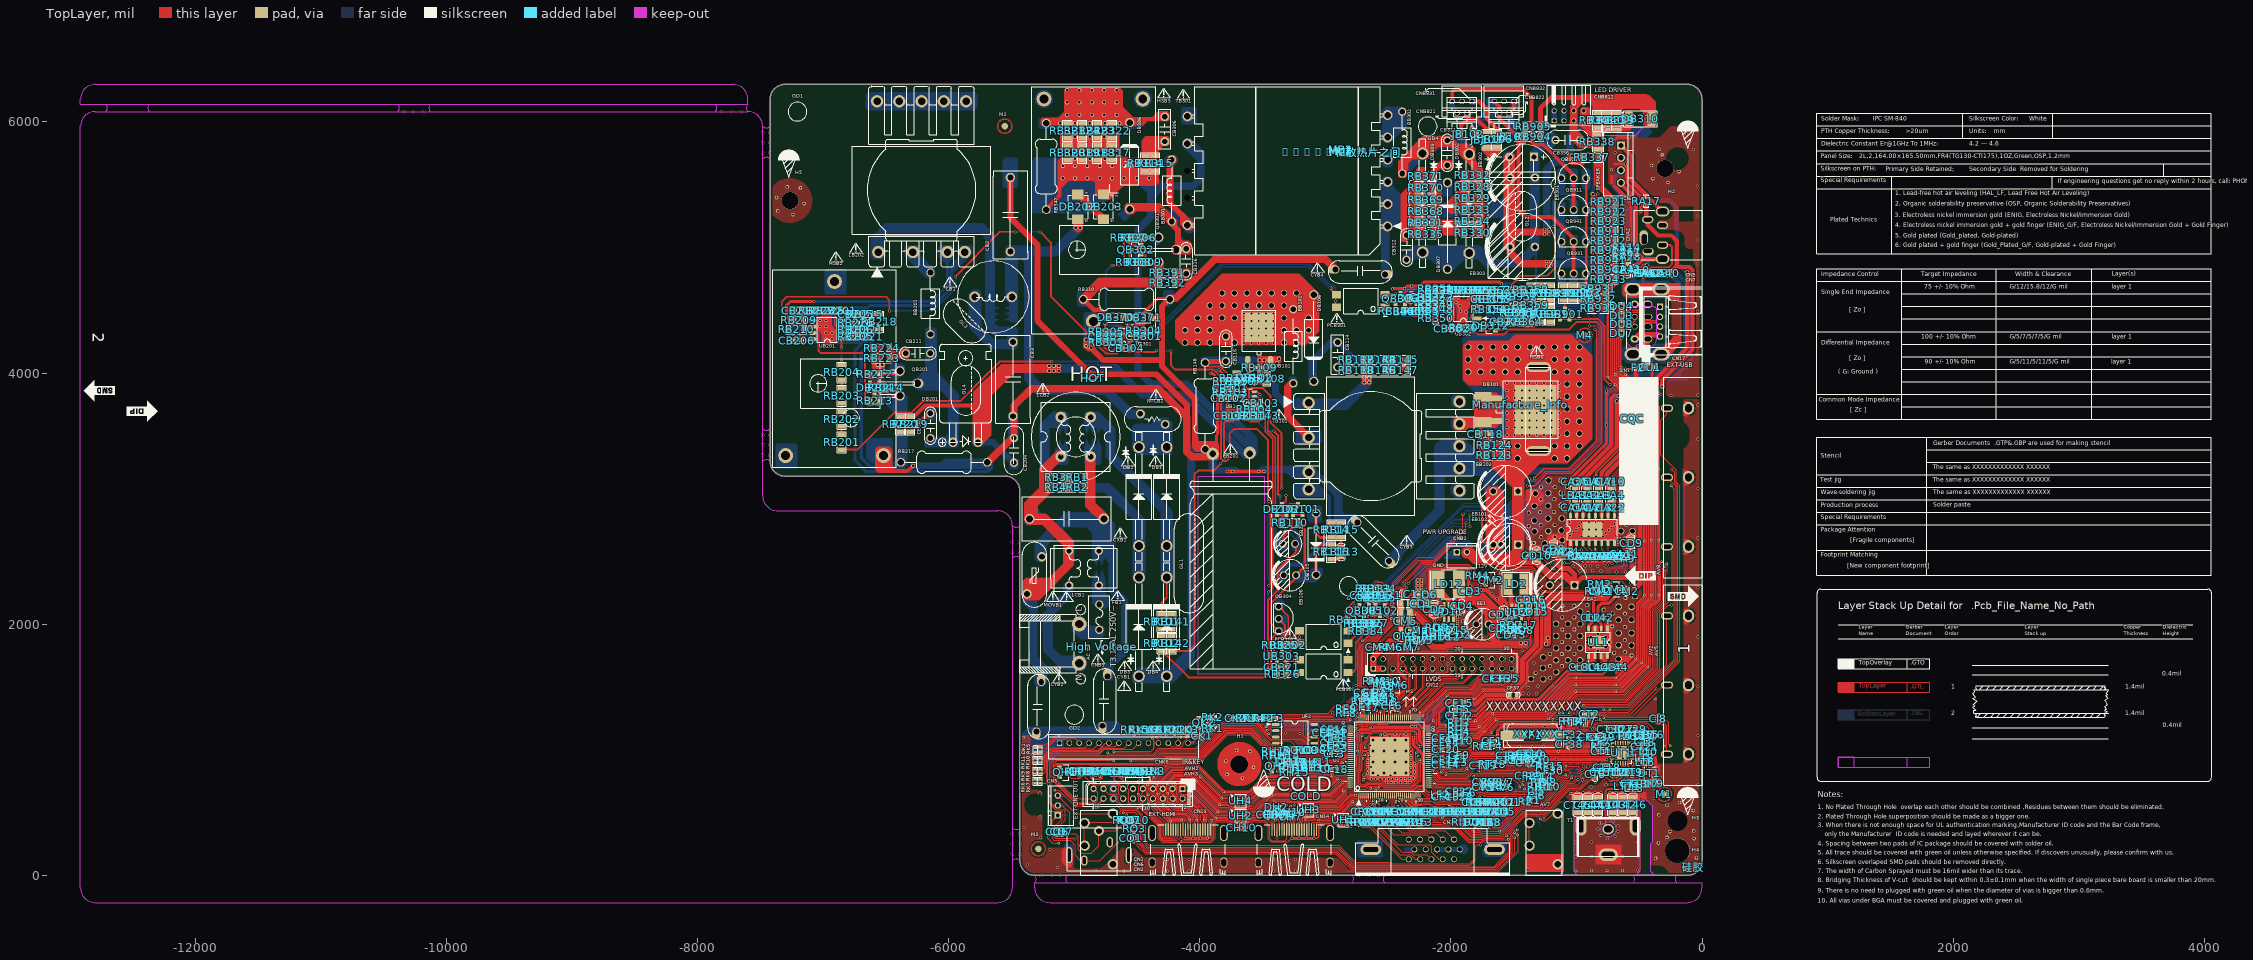
[diagram p0: TopLayer view]
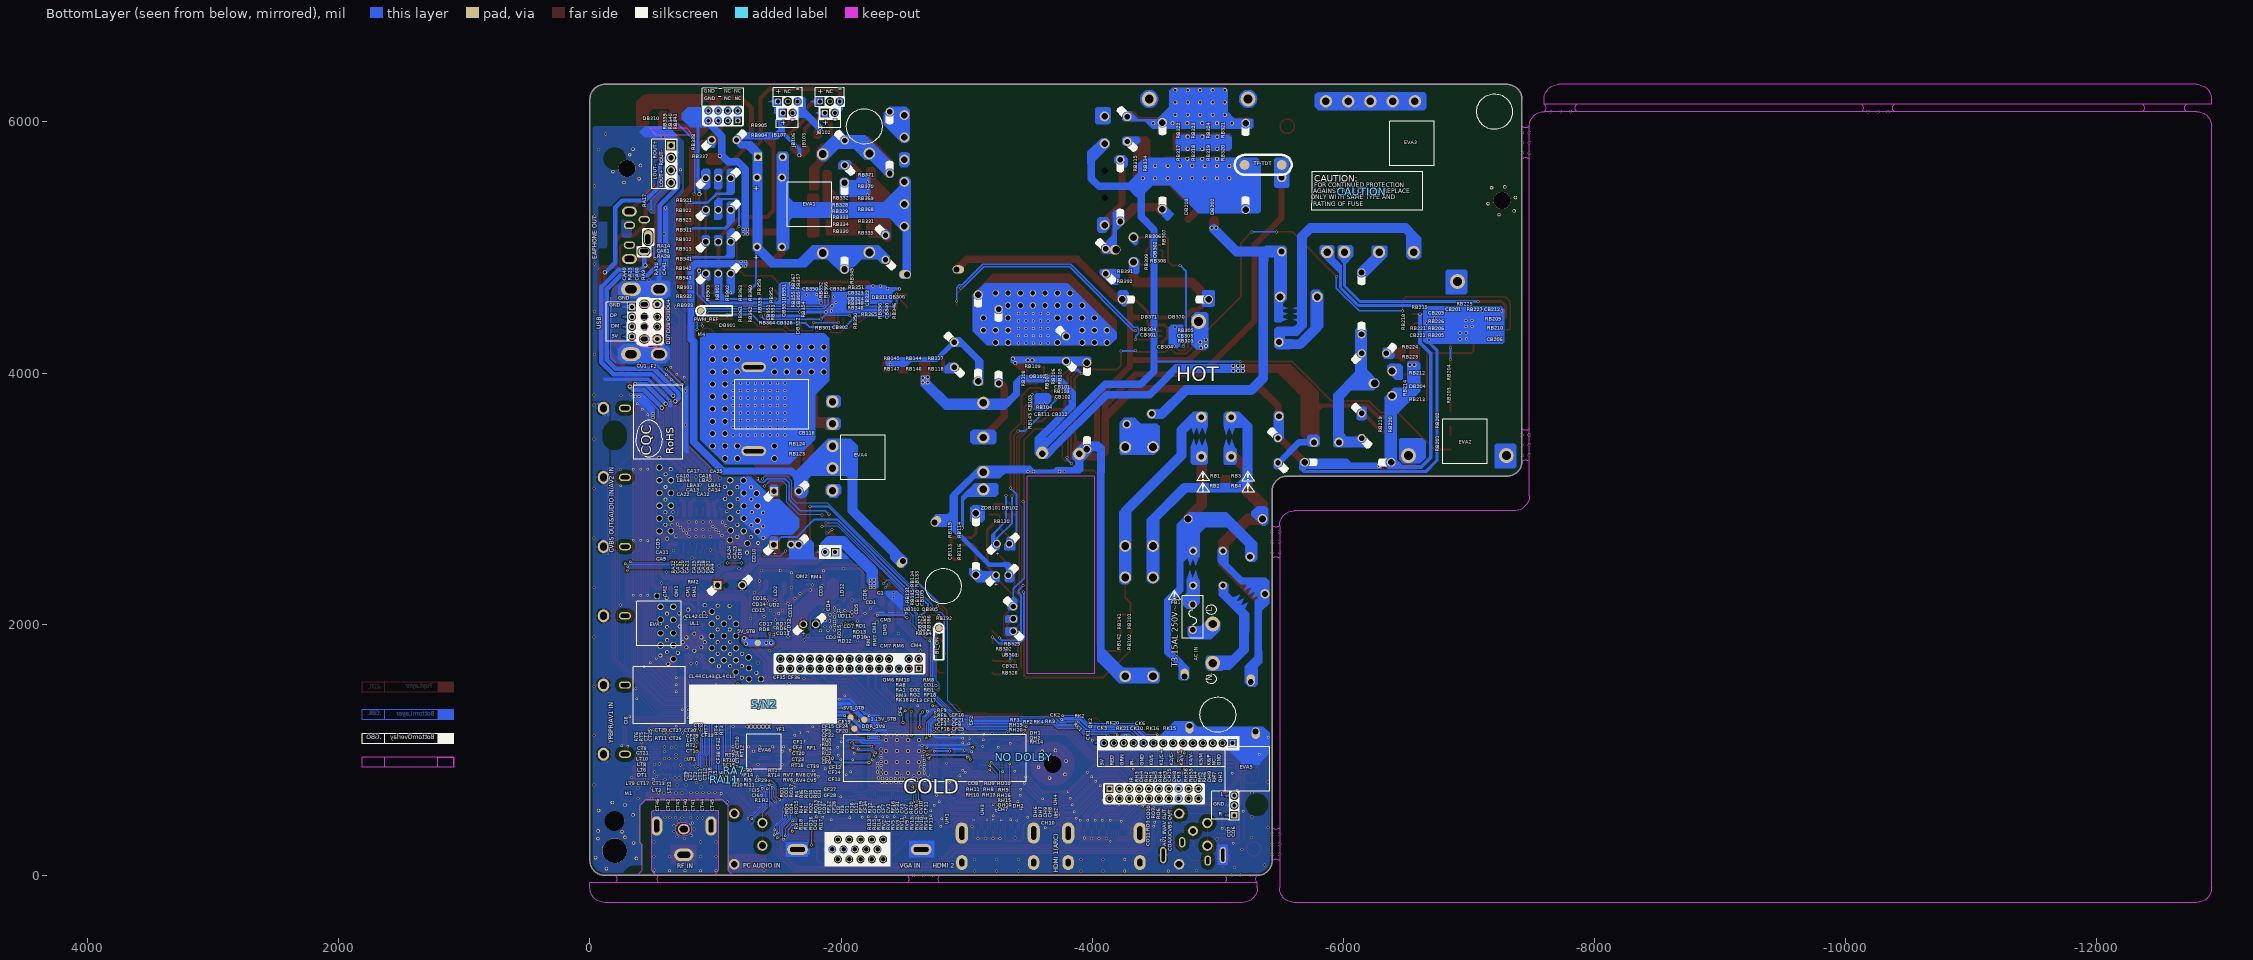
[diagram p1: BottomLayer view, seen from below]
# Altium PCB MISC84277.PcbDoc (part 1 of 15)
Units mil, origin at the board's own origin, x right, y up, seen from the top; angles counter-clockwise.
Board outline 7422.08 x 6299.21 mil, 2 copper layers (TopLayer, BottomLayer), stack 61.855 mil thick; 709 components, 395 nets, 2812 pads, 811 vias.

## Layer stack, top to bottom
TopSolder: solder mask 0.4, Solder Resist, Dk 3.5
TopLayer: signal copper 1.4
Dielectric1: core 59.055, FR-4, Dk 4.8
BottomLayer: signal copper 1.4
BottomSolder: solder mask 0.4, Solder Resist, Dk 3.5

## Board outline
-7304.33,3179.13 cw(c-7304.33,3297.24) -7422.44,3297.24 -7422.44,6181.1 cw(c-7304.33,6181.1) -7304.33,6299.21 -118.47,6299.21 cw(c-118.48,6181.1) -0.37,6181.1 -0.37,118.11 cw(c-118.48,118.11) -118.48,0 -5315.33,0 -5315.33,0.15 cw(c-5315.33,118.26) -5433.44,118.26 -5433.44,3061.02 ccw(c-5551.55,3061.02) -5551.55,3179.13

## Design rules (kind name [scope] priority, off if disabled: settings)
Clearance ■Poly_6.2mil [InPolygonClass('Poly_6.2mil') vs Not InPoly] p1: gap=6.2
Clearance ■KEEPOUT_18mil [(IsTrack Or IsArc) And (AsMM(Width) < 1) And IsKeepOut vs Not IsPad] p2: gap=18
Clearance ■HOT_7.2mm [InNetClass('HOT') vs InNetClass('All Nets') And (Not InNetClass('HOT'))] p3: gap=283.46
Clearance ■DFM_NPTH_10mil [IsPadHoleValid And (PadIsPlated=false) Or IsPad And (((AsMM(PadXSize_AllLayers) < 1) or (AsMM(PadYSize_AllLayers) < 1 ))) And IsKeepout vs Not IsPad] p4: gap=10
Clearance ■DFM_20mil [(IsTrack or IsArc or IsPad) And IsKeepOut vs IsTrack or IsArc or InPoly] p5: gap=20
Clearance ■PWR_A12_8mil [(InNetClass('PWR_A12_8mil') or InNet('*12V*') or InNet('*24V*') or InNet('*PVCC*') or InNet('*19V*') or InNet('*AMP*POWER*') or InNet('*AMP*VCC*') or InNet('*LNB*')) and Not IsPad vs Not InPoly] p6: gap=8
Clearance ■PS_L2All_3.2mm [InNet('L-1') vs InNet('*')] p7: gap=125.98
Clearance ■PS_L2LN_1.5mm [InNet('L') Or InNet('L-2') Or InNet('L-3') Or InNet('L-4') Or InNet('L-5') Or InNet('L-6') vs InNet('L-N') And Not(InNet('L') Or InNet('L-2') Or InNet('L-3') Or InNet('L-4') Or InNet('L-5') Or InNet('L-6'))] p8: gap=59.06
Clearance ■PS_N2LN_1.5mm [InNet('N') OR InNet('N-1') OR InNet('N-2') OR InNet('N-3') OR InNet('N-4') OR InNet('N-5') OR InNet('N-6') vs InNet('L-N') And Not (InNet('N') OR InNet('N-1') OR InNet('N-2') OR InNet('N-3') OR InNet('N-4') OR InNet('N-5') OR InNet('N-6'))] p9: gap=59.06
Clearance ■PS_L2LN_3mm [InNet('L') Or InNet('L-2') Or InNet('L-3') Or InNet('L-4') Or InNet('L-5') Or InNet('L-6') vs InNet('*') And Not (InNet('L-N') Or InNet('L') Or InNet('L-2') Or InNet('L-3') Or InNet('L-4') Or InNet('L-5') Or InNet('L-6') Or OnLayer('KeepOutLayer'))] p10: gap=118.11
Clearance ■PS_N2LN_3mm [InNet('N') OR InNet('N-1') OR InNet('N-2') OR InNet('N-3') OR InNet('N-4') OR InNet('N-5') OR InNet('N-6') vs InNet('*') And Not (InNet('L-N') Or InNet('N') OR InNet('N-1') OR InNet('N-2') OR InNet('N-3') OR InNet('N-4') OR InNet('N-5') OR InNet('N-6') Or OnLayer('KeepOutLayer'))] p11: gap=118.11
Clearance ■SIP2GND_8mil [HasFootprint('SIP*') vs InPoly] p12: gap=8
Clearance ■Poly_4mil [InPolygonClass('Poly_4mil') vs Not InPoly] p13: gap=4
Clearance ■Poly_5mil [InPolygonClass('Poly_5mil') vs Not InPoly] p14: gap=5
Clearance ■Poly_8mil [InPolygonClass('Poly_8mil') vs Not InPoly] p15: gap=8
Clearance ■ESD_10mil [HasFootprint('*IEC*') Or HasFootprint('*-F1*') Or HasFootprint('ANT-RF*')] p16: gap=10
Clearance ■ESD_20mil [HasFootprint('*SHIELD*')] p17: gap=20
Clearance ■C_RFGND_1.8mm [InNet('RFGND') vs Not (InNet('RF*IN*') OR InNet('NetCT40*'))] p18: gap=70.87
Clearance ■GND_12mil [InNet('GND') vs InPoly] p19: gap=12
Clearance ■ESD_30mil [(HasFootprint('SCART*') OR HasFootprint('AV*') OR HasFootprint('DB15*') OR HasFootprint('PHONE*')) vs OnBottomLayer] p20: gap=30
Clearance ■ESD_NT_30mil [HasFootprint('SCART*') Or HasFootprint('PHONE-HD-12') Or HasFootprint('PHONE-HD-17') Or HasFootprint('PHONE-HD-10') Or HasFootprint('PHONE-HD-26') vs InNet('GND') And OnTopLayer] p21: gap=30
Clearance ■DFM_TH_5mil [HasFootprint('GND') or HasFootprint('TP*') or HasFootprint('MARK*') or HasFootprint('SPARK_GAP') or HasFootprint('USB-HD-3-2') or HasFootprint('PHONE-HS-20') and Not IsRegion vs OnBottomlayer And IsPad OR IsPadHoleValid] p22: gap=5
Clearance ■DFM_HS60_5mil [InPadClass('HS60') vs InPadClass('HS60') OR IsPadHoleValid and not InPadClass('VIA5')] p23: gap=5
Clearance ■DFM_BCR_4mm [IsPadHoleValid vs IsBoardCutoutRegion] p24: gap=157.48
Clearance ■DFM_TH_4mm [OnBottomlayer And IsSMTPin vs IsPadHoleValid and not InPadClass('VIA5')] p25: gap=157.48
Clearance ■DFM_HS60_4mm [InPadClass('HS60') vs IsPad and OnBottomlayer] p26: gap=157.48
Clearance ■VIA2VIA_6.2mil [(IsVia OR InPadClass('VIA5')) And Not (IsVia And (AsMM(HoleDiameter) = 0.1)) vs (IsVia OR InPadClass('VIA5')) And Not (IsVia And (AsMM(HoleDiameter) = 0.1))] p27: gap=6.2
Clearance ■VIA2VIA_10.2mil [(IsVia OR InPadClass('VIA5')) And Not (IsVia And (AsMM(HoleDiameter) = 0.1)) vs (IsVia OR InPadClass('VIA5')) And Not (IsVia And (AsMM(HoleDiameter) = 0.1))] p28: gap=10.2
Clearance ■VIA2PAD_BGA_5mil [HasFootprint('BGA*') and IsPad vs (IsVia OR InPadClass('VIA5')) And Not (IsVia And (AsMM(HoleDiameter) = 0.1))] p29: gap=5
Clearance ■VIA2PAD_6mil [IsVia And Not (IsVia And (AsMM(HoleDiameter) = 0.1)) vs IsPad and Not HasFootprintPad('*','EPAD') and Not HasFootprintPad('*','257') and Not HasFootprintPad('TP','*') and Not HasFootprintPad  ('GND','JP*') and Not HasFootprintPad('LQFP216/0.4-2','217') and Not HasFootprintPad('QFP16*','17') and Not HasFootprintPad('QFN16*','17')  and Not HasFootprintPad('QFN20*','21') and Not HasFootprintPad('QFN24*','25') and Not HasFootprintPad( 'QFN24*','29') and Not  HasFootprintPad('QFN28*','29') and Not HasFootprintPad('QFN32*','33') and Not HasFootprintPad('QFN36*','37') and Not HasFootprintPad  ('QFN36*','0') and Not HasFootprintPad('QFN32*','0') and Not HasFootprintPad('QFN40*','41') and Not HasFootprintPad('QFN48*','49') and Not  HasFootprintPad('LQFP48/0.5-2','49') and Not HasFootprintPad('*SSOP32*','33') and Not HasFootprintPad('SOP8*','9') and Not HasFootprintPad  ('WSON8/1.27*','9') and Not HasFootprintPad('DFN10/0.5-1*','11') and Not HasFootprintPad('SON16/0.4','9') and Not HasFootprintPad  ('MSOP10/0.5-1','11') and Not HasFootprintPad('QFN56/0.5','57') and Not HasFootprintPad('LGA31/0.5','3*') and Not InPadClass('VIA_HS60')  and Not HasFootprintPad('TSSOP16/0.65-3','17') and Not HasFootprintPad('QFP128/0.5-2','129') and Not HasFootprintPad('QFP128/0.4-5','129')  and Not HasFootprintPad('PQFP48*','49') and Not HasFootprintPad('QFP156/0.4-1','157')] p30: gap=6
Clearance ■PAD2VIA5_6mil [IsPad And ((AsMM(PadXSize_AllLayers) < 2.5) or ((AsMM(PadYSize_AllLayers) < 2.5))) And Not InPadclass('HS60') vs InPadClass('VIA5')] p31: gap=6
Clearance "■12mil for Polygon" [InPoly] p32: gap=12
Clearance 8mil [All] p33 off: gap=8
Clearance 7mil [All] p34 off: gap=7
Clearance 6.2mil [All] p35 off: gap=6.2
Clearance 6mil [All] p36 off: gap=6
Clearance 5.8mil [All] p37 off: gap=5.8
Clearance 5mil [Not ((IsTrack Or IsArc) And (Layer = 'KeepOutLayer')) vs Not (IsPad or ((IsTrack Or IsArc) And (Layer = 'KeepOutLayer')))] p38: gap=5
Clearance 4.5mil [Not ((IsTrack Or IsArc) And (Layer = 'KeepOutLayer')) vs Not (IsPad or ((IsTrack Or IsArc) And (Layer = 'KeepOutLayer')))] p39 off: gap=4.5
Clearance "4mil for Minimum" [Not ((IsTrack Or IsArc) And (Layer = 'KeepOutLayer')) vs Not (IsPad or ((IsTrack Or IsArc) And (Layer = 'KeepOutLayer')))] p40 off: gap=4
ComponentClearance [All] p1 off: gap=0.1 collisioncheckmode=3 verticalgap=39.37 showdistances=FALSE
DiffPairsRouting DiffPair_USB_DiffPairsRouting [InDifferentialPairClass('USB')] p1: maxlimit=5 minlimit=4 mostfreqgap=5 toplayer_minwidth=15 toplayer_maxwidth=15 toplayer_prefwidth=15 bottomlayer_minwidth=15 bottomlayer_maxwidth=15 bottomlayer_prefwidth=15 maxuncoupledlength=200
DiffPairsRouting DiffPair_LVDS_DiffPairsRouting [InDifferentialPairClass('LVDS')] p2: maxlimit=5 minlimit=4 mostfreqgap=5 toplayer_minwidth=15 toplayer_maxwidth=15 toplayer_prefwidth=15 bottomlayer_minwidth=15 bottomlayer_maxwidth=15 bottomlayer_prefwidth=15 maxuncoupledlength=500
DiffPairsRouting DiffPair_HDMI_DiffPairsRouting [InDifferentialPairClass('HDMI')] p3: maxlimit=5 minlimit=4 mostfreqgap=5 toplayer_minwidth=15 toplayer_maxwidth=15 toplayer_prefwidth=15 bottomlayer_minwidth=15 bottomlayer_maxwidth=15 bottomlayer_prefwidth=15 maxuncoupledlength=200
DiffPairsRouting [All] p4: maxlimit=10 minlimit=10 mostfreqgap=10 toplayer_minwidth=15 toplayer_maxwidth=15 toplayer_prefwidth=15 bottomlayer_minwidth=15 bottomlayer_maxwidth=15 bottomlayer_prefwidth=15 maxuncoupledlength=500
FabricationTestPointUsage TestPointUsage [All] p1: valid=0 allowmultiple=FALSE
FabricationTestpoint Testpoint [All] p1: side=3 testpointundercomponent=TRUE minsize=40 maxsize=100 preferedsize=60 minholesize=20 maxholesize=40 preferedholesize=32 testpointgrid=1 allowsidetop=TRUE allowsidebottom=TRUE usegrid=TRUE gridtolerance=0.01
HoleSize HoleSize_VIA [ISVIA] p1 off: absolutevalues=TRUE maxlimit=23.62 minlimit=7.87 maxpercent=80.000 minpercent=20.000
HoleToHoleClearance Hole2Hole [All] p1 off: gap=18 allowstackedmicrovias=FALSE
MatchedLengths DiffPair_USB_MatchedLengths [InDifferentialPairClass('USB')] p1: tolerance=100 checknetsindiffpair=TRUE checkdiffpairvsdiffpair=TRUE checkothers=TRUE
MatchedLengths DiffPair_LVDS_MatchedLengths [InDifferentialPairClass('LVDS')] p2: tolerance=100 checknetsindiffpair=TRUE checkdiffpairvsdiffpair=TRUE checkothers=TRUE
MatchedLengths DiffPair_HDMI_MatchedLengths [InDifferentialPairClass('HDMI')] p3: tolerance=100 checknetsindiffpair=TRUE checkdiffpairvsdiffpair=TRUE checkothers=TRUE
MinimumAnnularRing [All] p1: minimumring=3.94
MinimumSolderMaskSliver [All] p1 off: minsoldermaskwidth=-1
NetAntennae [Not (HasFootprint('ANT-7') or HasFootprint('ANT-BLUECORE'))] p1: netantennaetolerance=40
PermittedLayers [All] p1: toplayerpermitted=TRUE bottomlayerpermitted=TRUE
PlaneClearance Plane_ESD_30mil [(HasFootprint('SCART*') OR HasFootprint('AV*') OR HasFootprint('DB15*') OR HasFootprint('PHONE*'))] p1: clearance=30
PlaneClearance [All] p2: clearance=9
PlaneConnect Plane2Via [IsVia or InPadClass('VIA5')] p1: planeconnectstyle=Direct reliefexpansion=20 reliefentries=4 reliefconductorwidth=10 reliefairgap=10
PlaneConnect PlaneConnect_PAD [HasFootprint('ASSE*') OR InPadclass('HS60')] p2: planeconnectstyle=Direct reliefexpansion=20 reliefentries=4 reliefconductorwidth=10 reliefairgap=10
PlaneConnect [All] p3: planeconnectstyle=Relief reliefexpansion=12 reliefentries=4 reliefconductorwidth=30 reliefairgap=12
PolygonConnect PourOverVia [IsVia vs IsPolygon] p1: connectstyle=Direct reliefconductorwidth=10 reliefentries=4 polygonreliefangle="90 Angle" airgapwidth=10
PolygonConnect VIA5_HS60 [InPadclass('HS60') or InPadClass('VIA5') vs IsPolygon] p2: connectstyle=Direct reliefconductorwidth=10 reliefentries=4 polygonreliefangle="90 Angle" airgapwidth=10
PolygonConnect Polygon_RFGND [InNet('RFGND')] p3: connectstyle=Direct reliefconductorwidth=10 reliefentries=4 polygonreliefangle="90 Angle" airgapwidth=10
PolygonConnect ESD_SCART [HasFootprint('SCART*') vs IsPolygon And onBottomlayer] p4: connectstyle=Direct reliefconductorwidth=30 reliefentries=4 polygonreliefangle="90 Angle" airgapwidth=10
PolygonConnect FH2Polygon [HasFootprint('ASSE*') or HasFootprint('DIODE-S0402') vs IsPolygon] p5: connectstyle=Direct reliefconductorwidth=10 reliefentries=4 polygonreliefangle="90 Angle" airgapwidth=10
PolygonConnect PWC1_2Polygon [(HasFootprint('*0805*') OR HasFootprint('*1206*')) vs IsPolygon] p6: connectstyle=Relief reliefconductorwidth=30 reliefentries=4 polygonreliefangle="90 Angle" airgapwidth=10
PolygonConnect PWC2_2Polygon [HasFootprint('*0603*') vs IsPolygon] p7: connectstyle=Relief reliefconductorwidth=25 reliefentries=4 polygonreliefangle="90 Angle" airgapwidth=10
PolygonConnect PWC3_2Polygon [HasFootprint('EC*') vs IsPolygon] p8: connectstyle=Relief reliefconductorwidth=35 reliefentries=4 polygonreliefangle="90 Angle" airgapwidth=10
PolygonConnect PWC2Polygon [(HasFootprint('SOT-89') OR HasFootprint('SOT-223') OR HasFootprint('TO-252') OR HasFootprint('TO-263') OR HasFootprint('DIODE') OR HasFootprint('SW-HS-2') OR HasFootprint('HDMI*') OR HasFootprint('SO-8B') OR HasFootprint('GND') OR HasFootprint('PHONE*') OR HasFootprint('DIP18/2.54-2') OR HasFootprint('DIP18/2.54-1') OR HasFootprint('UFL-R-SMT-1') OR HasFootprint('WIFI') OR HasFootprint('UM02BS') OR HasFootprint('*SCART*') OR HasFootprint('TSOT23-8/0.65') OR HasFootprint('*SOT-23-*') OR HasFootprint('SOP23-5-1') OR HasFootprint('SOP6/0.95') OR HasFootprint('M-WIFI-2-M603USA1') OR HasFootprint('M-MT7632U') OR HasFootprint('SOP8/1.27') OR HasFootprint('SOP8/1.27-3')) vs IsPolygon] p9: connectstyle=Direct reliefconductorwidth=35 reliefentries=4 polygonreliefangle="90 Angle" airgapwidth=10
PolygonConnect SMD2Polygon [IsSMTPin vs IsPolygon] p10: connectstyle=Relief reliefconductorwidth=12 reliefentries=4 polygonreliefangle="90 Angle" airgapwidth=10
PolygonConnect PTH2Polygon [IsThruPin vs IsPolygon] p11: connectstyle=Relief reliefconductorwidth=25 reliefentries=4 polygonreliefangle="90 Angle" airgapwidth=10
RoutingVias 0.6_0.4 [All] p1 off: holewidth=15.75 width=23.62 viastyle="Through Hole" minholewidth=15.75 minwidth=23.62 maxholewidth=15.75 maxwidth=23.62
RoutingVias 0.8_0.5 [All] p2 off: holewidth=19.68 width=31.5 viastyle="Through Hole" minholewidth=19.68 minwidth=31.5 maxholewidth=19.68 maxwidth=31.5
RoutingVias 0.5_0.3 [All] p3: holewidth=11.81 width=19.68 viastyle="Through Hole" minholewidth=11.81 minwidth=19.68 maxholewidth=11.81 maxwidth=19.68
RoutingVias 0.45_0.25 [All] p4 off: holewidth=9.84 width=17.72 viastyle="Through Hole" minholewidth=9.84 minwidth=17.72 maxholewidth=9.84 maxwidth=17.72
RoutingVias 0.4_0.2 [All] p5 off: holewidth=7.87 width=15.75 viastyle="Through Hole" minholewidth=7.87 minwidth=15.75 maxholewidth=7.87 maxwidth=15.75
RoutingVias 0.25_0.1 [All] p6 off: holewidth=3.94 width=9.84 viastyle="Through Hole" minholewidth=3.94 minwidth=9.84 maxholewidth=3.94 maxwidth=9.84
SMDNeckDown SMDNeckDown_Chip [HasFootprint('FFC*') or HasFootprint('QFP*') or HasFootprint('QFN*') or HasFootprint('HDMI*') or HasFootprint('BGA*')] p1: percent=100.000
SMDToCorner [All] p1 off: distance=40000
ShortCircuit ■ShortCircuit_ViaOnEpad [HasFootprintPad( '*','EPAD') vs IsVia AND InNet('*')] p1: allowed=TRUE
ShortCircuit ■ShortCircuit_JP [HasFootprintPad( 'GND','JP_1K') vs HasFootprintPad( 'GND','JP_2K')] p2: allowed=TRUE
ShortCircuit ■ShortCircuit_0402 [HasFootprintPad('R0402SC','1') Or HasFootprintPad('R0402SC','2') vs HasFootprintPad('R0402SC','3')] p3: allowed=TRUE
ShortCircuit ■ShortCircuit [InNet('*')] p4: allowed=FALSE
SilkToSilkClearance Silk2Silk [All] p1: silktosilkclearance=0.1
SilkToSolderMaskClearance SilkscreenOverComponentPads [IsText] p1: minsilkscreentomaskgap=0.1 clearancetoexposedcopper=TRUE
SolderMaskExpansion SolderMask_VIA [IsVia] p1: expansion=5.1
SolderMaskExpansion [All] p2: expansion=3
UnRoutedNet ■UnRoutedNet [All] p1:
ViasUnderSMD [All] p1: allowed=FALSE
Width DiffPair_USB_Width [InDifferentialPairClass('USB')] p1: maxlimit=11 minlimit=4 preferedwidth=11
Width DiffPair_LVDS_Width [InDifferentialPairClass('LVDS')] p2: maxlimit=7 minlimit=4 preferedwidth=7
Width DiffPair_HDMI_Width [InDifferentialPairClass('HDMI')] p3: maxlimit=7 minlimit=4 preferedwidth=7
Width [All] p4: maxlimit=250 minlimit=3 preferedwidth=8
16 further rules are at their usual default settings.

## Classes and differential pairs
net class HOT: 380V BRO BRO1 COMP CS D H L L-1 L-2 L-3 L-N N-1 N-2 N-3 NetBB101_2 NetBB201_1 NetBB201_2 NetBB301_1 NetCB3_1 NetCB101_1 NetCB102_1 NetCB103_1 NetCB111_2 NetCB113_1 NetCB113_2 NetCB114_1 NetCB114_2 NetCB116_1 NetCB201_2 NetCB206_2 NetCB209_1 NetCB211_2 NetCB212_1 NetCB221_2 NetCB306_1 NetCB306_2 NetCB316_1 NetCB321_1 NetCB321_2 NetDB1_K NetDB102_1 NetDB108_K NetDB202_K NetDB204_1 NetDB204_2 NetDB370_A NetDB370_K NetPCB303_4 NetQB101_G NetQB102_B NetQB102_C NetQB201_S NetQB301_G NetQB302_B NetQB302_C NetRB101_2 NetRB106_1 NetRB114_2 NetRB141_1 NetRB144_2 NetRB201_2 NetRB202_2 NetRB203_2 NetRB204_2 NetRB209_1 NetRB212_1 NetRB226_2 NetRB317_1 OUT PFC_CS SGND VBRIDGE VCC1 VCC2 ZCD
component class TV#07_Tuner: CT1 CT2 CT5 CT6 CT7 CT8 CT9 CT10 CT11 CT12 CT13 CT17 CT18 CT19 CT20 CT21 CT23 CT24 CT25 CT26 CT27 CT29 CT30 CT40 CT41 CT42 CT43 CT44 CT45 CT46 DT1 LT1 LT2 LT3 LT6 LT8 LT9 LT10 LT11 RT1 RT2 RT4 RT5 RT6 RT7 RT9 RT10 RT11 RT12 RT14 RT18 T1 UT1
component class TV#06_AMP: CA9 CA10 CA11 CA12 CA13 CA14 CA15 CA16 CA17 CA18 CA19 CA20 CA21 CA22 CA23 CA24 CA25 CA31 CA32 CA40 CA41 CA60 CA61 CD8 CD9 CD10 CNA1 CNA2 EA1 LBA1 LBA2 LBA3 LBA4 RA1 RA4 RA7 RA8 RA9 RA10 RA11 RA12 RA14 RA17 RA23 RA28 UA1
component class TV#05_HDMI: AVH2 AVH3 CH3 CH4 CH7 CH8 CH9 CH10 CH15 CN13 CN14 DH1 DH2 DH3 DH4 DH5 DH6 DH7 DH8 DH9 DH10 QH1 QH2 RH1 RH2 RH3 RH4 RH5 RH6 RH7 RH8 RH9 RH10 RH11 RH13 RH14 RH15 RH16 RH19 RH20 RH55 RH56 UH1 UH2 UH3 UH4
component class TV#04_INPUT: AV2 AV5 AV7 AV8 CI1 CI2 CI3 CI4 CI5 CI6 CI7 CI8 CI9 CI11 CN1 CN2 CN3 CN5 CN6 CN7 CN11 CN17 CO1 CO4 CO6 CO7 CO8 CO9 CO10 CO11 CU1 CV1 CV3 CV5 CV6 CV7 CV9 CV10 DU1 DU3 DU4 DU7 DU8 F2 R1 R2 R3 R4 RI1 RI2 RI3 RI4 RI5 RI6 RI7 RI8 RI9 RI10 RI11 RI12 RI13 RI14 RI15 RI16 RI17 RI18 RO1 RO2 RO3 RO5 RO6 RO7 RO9 RO10 RO12 RO13 RO15 RO16 RO17 RU1 RU2 RU3 RU4 RV1 RV2 RV3 RV4 RV5 RV6 RV7 RV8 RV9 RV10 RV11 RV12 RV13 RV14
component class TV#03_TSUMV56: CF1 CF2 CF3 CF4 CF5 CF6 CF7 CF8 CF9 CF10 CF11 CF12 CF13 CF14 CF15 CF16 CF17 CF18 CF19 CF20 CF21 CF22 CF23 CF24 CF25 CF26 CF27 CF28 CF29 CF30 CF31 CF32 CF33 CF34 CF35 CF36 CF37 CF38 CF39 CF40 CK1 CK2 CK3 CK6 CK10 CN12 CNK6 DK1 LF1 LF2 LF3 LF4 LF5 LF6 LF7 QK2 RF1 RF2 RF3 RF8 RF9 RF10 RF11 RF12 RF13 RF14 RF15 RF16 RF18 RF19 RF24 RK1 RK2 RK3 RK4 RK5 RK6 RK7 RK8 RK9 RK10 RK11 RK15 RK16 RK18 RK20 RK21 RT3 RT4 U1 UF2 YF1
component class TV#02_POWER: 1.15V_STB 3V3_STB 5V_STB C1 CD1 CD2 CD3 CD4 CD5 CD6 CD7 CD11 CD12 CD13 CD14 CD15 CD16 CD17 CG1 CG2 CL2 CL3 CL4 CL42 CL43 CL44 CM1 CM2 CM3 CM4 CM5 CM7 DDR_1V8 EE1 LD2 LD12 QM1 QM2 QM5 QM6 R5V R12V RD1 RD6 RD7 RD8 RD12 RD13 RD15 RD16 RG1 RG2 RM1 RM2 RM3 RM4 RM5 RM6 RM7 RM8 RM10 UD2 UD11 UL1
component class PS#01_XXXXXXXXXXXX: BB101 BB201 BB301 BB302 BL_ON CB2 CB3 CB101 CB102 CB103 CB109 CB110 CB111 CB112 CB113 CB114 CB116 CB118 CB201 CB204 CB205 CB206 CB209 CB211 CB212 CB221 CB301 CB302 CB303 CB304 CB305 CB306 CB311 CB312 CB316 CB321 CB322 CB323 CB324 CB326 CB327 CB328 CB340 CB350 CB356 CB951 CNB1 CNB2 CNB812 CNB821 CNB822 CNB831 CNB832 CXB1 CYB1 CYB2 CYB3 CYB4 DB1 DB2 DB3 DB4 DB101 DB102 DB105 DB106 DB108 DB109 DB201 DB202 DB203 DB204 DB302 DB303 DB306 DB307 DB310 DB311 DB312 DB370 DB371 DB901 DB951 EB101 EB102 EB103 EB106 EB107 EB201 EB301 EB302 EB303 EVA1 EVA2 EVA3 EVA4 EVA5 EVA6 EVA7 FB1 GD1 GD2 GD3 GD4 GL1 GL2 GL3 GL4 HSB2 HSB3 HSB6 JB102 JB103 JB106 JB107 LB1 LB202 LCB1 LCB2 MB1 MB2 ML1 MOVB1 NTCB2 PCB101 PCB301 PCB303 PWM_REF QB101 QB102 QB201 QB201和散热片之间 QB301 QB301和散热片之间 QB302 QB304 QB305 QB306 QB911 QB921 QB931 QB941 QB951 RB1 RB2 RB3 RB4 RB101 RB102 RB103 RB104 RB105 RB106 RB107 RB108 RB109 RB110 RB114 RB115 RB116 RB117 RB118 RB123 RB124 RB131 RB132 RB133 RB134 RB135 RB141 RB142 RB143 RB144 RB145 RB146 RB147 RB148 RB201 RB202 RB203 RB204 RB205 RB206 RB209 RB210 RB212 RB213 RB214 RB215 RB217 RB218 RB219 RB220 RB221 RB223 RB224 RB225 RB226 RB227 RB301 RB302 RB303 RB304 RB305 RB306 RB307 RB308 RB309 RB310 RB314 RB315 RB317 RB318 RB319 RB320 RB321 RB322 RB323 RB324 RB325 RB326 RB328 RB329 RB330 RB331 RB332 RB333 RB334 RB335 RB337 RB338 RB339 RB340 RB341 RB345 RB346 RB347 RB348 RB349 RB350 RB351 RB352 RB354 RB355 RB356 RB357 RB358 RB359 RB360 RB361 RB362 RB363 RB364 RB365 RB366 RB367 RB368 RB369 RB370 RB371 RB384 RB385 RB386 RB391 RB392 RB901 RB902 RB903 RB904 RB905 RB911 RB912 RB913 RB921 RB922 RB923 RB931 RB932 RB933 RB941 RB942 RB943 RB951 RB952 TB101 TB301 TP-TDT UB101 UB102 UB201 UB301 UB302 UB303 ZDB101
component class PCB_info: A13XX Barcode CAUTION COLD CQC DIP H1 H2 H3 H4 H5 "High Voltage" HOT HS M1 M2 M3 M4 Manufacture_Info "NO DOLBY" S/N1 S/N2 SMD XXXXXX XXXXXXXXXXXX 硅胶
pad class VIA5: CH7-1 CT41-2 CT43-2 Free-VIA5 UH1-GND UH2-GND UH3-GND UH4-GND
pad class ShortCricuit_JP2: GND_JP1-JP_2K GND_JP2-JP_2K
pad class ShortCricuit_JP1: GND_JP1-JP_1K GND_JP2-JP_1K
pad class HS60: Free-HS60
polygon class Poly_5mil: 5mil

## Components (designator, comment, footprint, x,y, rotation, side; value= is the part's Value field where it differs from the comment)
1.15V_STB "TEST" TP -2185,1240 r0 bottom
3V3_STB "TEST" TP -2076,1257 r90 bottom
5V_STB "TEST" TP -1337,1851.35 r90 bottom
AV2 "RCA terminal, RCA Jack, AV3, H, Yellow, White, Red, CH5.5, D14, Seal, DIP, RC075-F03L3BY-A, YUQIU (MI material)" AV3-H14-15 0,1515.75 r90 top locked
AV5 "NC/RCA terminal, RCA Jack, AV3, H, Green, Blue, Red, CH5.5, D14, Seal, DIP, RC075-F03L3BY-B, YUQIU (MI material)" AV3-H14-15 0,1515.75 r90 top locked
AV7 "Earphone terminal, Earphone Jack, H, Φ3.5, CH7.0, Black, Seal, DIP, PJ7723-F03L3BY-C, YUQIU" PHONE-HD-41 -1259.84,0 r0 top locked
AV8 "RCA terminal, RCA Jack, AV3, H, Yellow, White, Red, CH5.5, D14, Seal, DIP, RC075-F03L3BY-A, YUQIU (MI material)" AV3-H14-15 0,3169.29 r90 top locked
AVH2 "NC/NC/connect jack, 2×10Pin, D2.0, D, SNAP, Fool-proofing, Beige, L=2.6mm, DIP, CJ" SIP2*10/2.0D-4 -4492.15,650.33 r0 top locked
AVH3 "NC/gold pin, pin connector, 2×10Pin, D, D2.0mm, L=2.6mm, DIP, LK" SIP2*10/2.0DM-1 -4492.15,650.33 r0 top locked
BB101 "φ3.5×6.0×0.65mm-CP (tape and reel/Xiuyida)" LB/3.5*6*15 -3255.22,4214 r270 top
BB201 "φ3.5×6.0×0.65mm-CP (tape and reel/Xiuyida)" LB/3.5*6*12.5 -6145,4554.94 r270 top
BB301 "φ3.5×6.0×0.65mm-CP (tape and reel/Xiuyida)" LB/3.5*6*12.5 -4223.5,5454 r90 top
BB302 "φ3.5×6.0×0.65mm-CP (tape and reel/Xiuyida)" LB/3.5*6*12.5 -2387.5,5836 r270 top
BL_ON "TEST" TP_BL -2779.53,1968.5 r90 bottom
C1 "NC/10uF-1206-X5R-±10%-16V" C1206 -2320.87,2238.19 r0 top
CA9 "1000pF-0402-X7R-±10%-50V" C0402 -619,2521.98 r180 top
CA10 "2200pF-0402-X7R-±10%-50V" C0402 -728,3134.02 r0 top
CA11 "0.1uF-0402-X5R-±20%-16V" C0402 -619,2557.99 r180 top
CA12 "0.22uF-0402-X5R-±10%-16V" C0402 -920,2927 r180 top
CA13 "0.22uF-0402-X5R-±10%-16V" C0402 -827,2927.02 r0 top
CA14 "0.22uF-0402-X5R-±10%-16V" C0402 -1012,2927.02 r0 top
CA15 "1uF-0402-X5R-±20%-16V" C0402 -840.99,2540.5 r90 top
CA16 "2200pF-0402-X7R-±10%-50V" C0402 -920,3134.02 r180 top
CA17 "2200pF-0402-X7R-±10%-50V" C0402 -827,3134 r180 top
CA18 "0.22uF-0402-X5R-±10%-16V" C0402 -913.47,2540.5 r270 top
CA19 "0.22uF-0402-X5R-±10%-16V" C0402 -877.22,2540.5 r270 top
CA20 "0.22uF-0402-X5R-±10%-16V" C0402 -747.47,2540.5 r270 top
CA21 "0.22uF-0402-X5R-±10%-16V" C0402 -783.72,2540.5 r270 top
CA22 "0.22uF-0402-X5R-±10%-16V" C0402 -728,2927 r180 top
CA23 "0.1uF-0402-X5R-±20%-16V" C0402 -1131,2578 r90 top
CA24 "1000pF-0402-X7R-±10%-50V" C0402 -1095,2578 r90 top
CA25 "2200pF-0402-X7R-±10%-50V" C0402 -1012,3134 r180 top
CA31 "3300pF-0402-X7R-±10%-50V" C0402 -949.74,2540.5 r90 top
CA32 "3300pF-0402-X7R-±10%-50V" C0402 -711.22,2540.5 r270 top
CA40 "10uF-0805-X5R-±20%-16V" C0805 -294.29,4796.5 r0 top
CA41 "10uF-0805-X5R-±20%-16V" C0805 -598.3,4827.4 r270 top
CA60 "6800pF-0402-X7R-±10%-50V" C0402 -419.79,4796.49 r270 top
CA61 "6800pF-0402-X7R-±10%-50V" C0402 -600.22,4961.5 r180 top
CAUTION "CAUTION" CAUTION -6148.05,5442.42 r180 bottom
CB2 "B32672P4474K006(EPCOS)" CAP18*7-V-15 -5509,5262.5 r90 top
CB3 "B32672P4474K006(EPCOS)" CAP18*7-V-15 -5488,3951.5 r270 top
CB101 "100pF-0402-NPO-±5%-50V" C0402 -3759.5,3879.5 r180 top
CB102 "0.1uF-0603-X7R-±10%-50V" C0603 -3768.5,3798 r180 top
CB103 "1000pF-0402-X7R-±10%-50V" C0402 -3513,3760 r270 top
CB109 "0.1uF-0603-X7R-±10%-50V" C0603 -2661.42,2230.31 r90 top
CB110 "NC/1000pF-0402-X7R-±10%-50V" C0402 -2618.12,2210.63 r90 top
CB111 "NC/1uF-0805-X7R-±10%-25V" C0805 -3602.5,3660 r180 top
CB112 "NC/1uF-0805-X7R-±10%-25V" C0805 -3744,3660.5 r0 top
CB113 "220PF-0805-NPO-±10%-200V" C0805 -2875.84,2575.32 r270 top
CB114 "C242G472J20A201 (tape and reel/Faraday)" CAP8*2.5-V-5 -2902.49,4146.36 r90 top
CB116 "Ceramic capacitor, CAP CD, 1KV, 100pF, ±10%, SL, P, 5.0mm, DIP, TP, SHM" CAP7.5*2.5-V-5 -3792,4193.5 r90 top locked
CB118 "1000pF-0805-NPO-±10%-200V" C0805 -1727.5,3511.5 r0 top
CB201 "0.047uF-0603-X7R-±10%-25V" C0603 -6874.48,4496.35 r180 top
CB204 "NC/ceramic capacitor, CAP CD, 1KV, 4700pF, ±20%, Y5U, P, 5.0mm, DIP, TP, TongHao" CAP9.8*4-V-5 -5480.13,3384.94 r270 top
CB205 "220pF-0402-NPO-±5%-50V" C0402 -6741.19,4468.79 r180 top
CB206 "0.1uF-0603-X7R-±10%-50V" C0603 -7209.84,4257.84 r0 top
CB209 "Ceramic capacitor, CAP CD, 1KV, 100pF, ±10%, SL, P, 5.0mm, DIP, TP, SHM" CAP7.5*2.5-V-5 -6146,3581.03 r270 top
CB211 "CC45SL3AD470JYPNA(TDK)" CAP7.5*2.5-V-5 -6245,4157 r180 top
CB212 "0.22uF-0805-X7R-±10%-50V" C0805 -7186.75,4496.35 r180 top
CB221 "4700pF-0402-X7R-±10%-50V" C0402 -6666.39,4290.01 r0 top
CB301 "4700pF-0402-X7R-±10%-50V" C0402 -4447.08,4295.33 r180 top
CB302 "Ceramic capacitor, CAP MC, 25V, 1uF, ±10%, X7R, 0603, SMD, TP" C0603 -1994.5,4354.5 r180 top